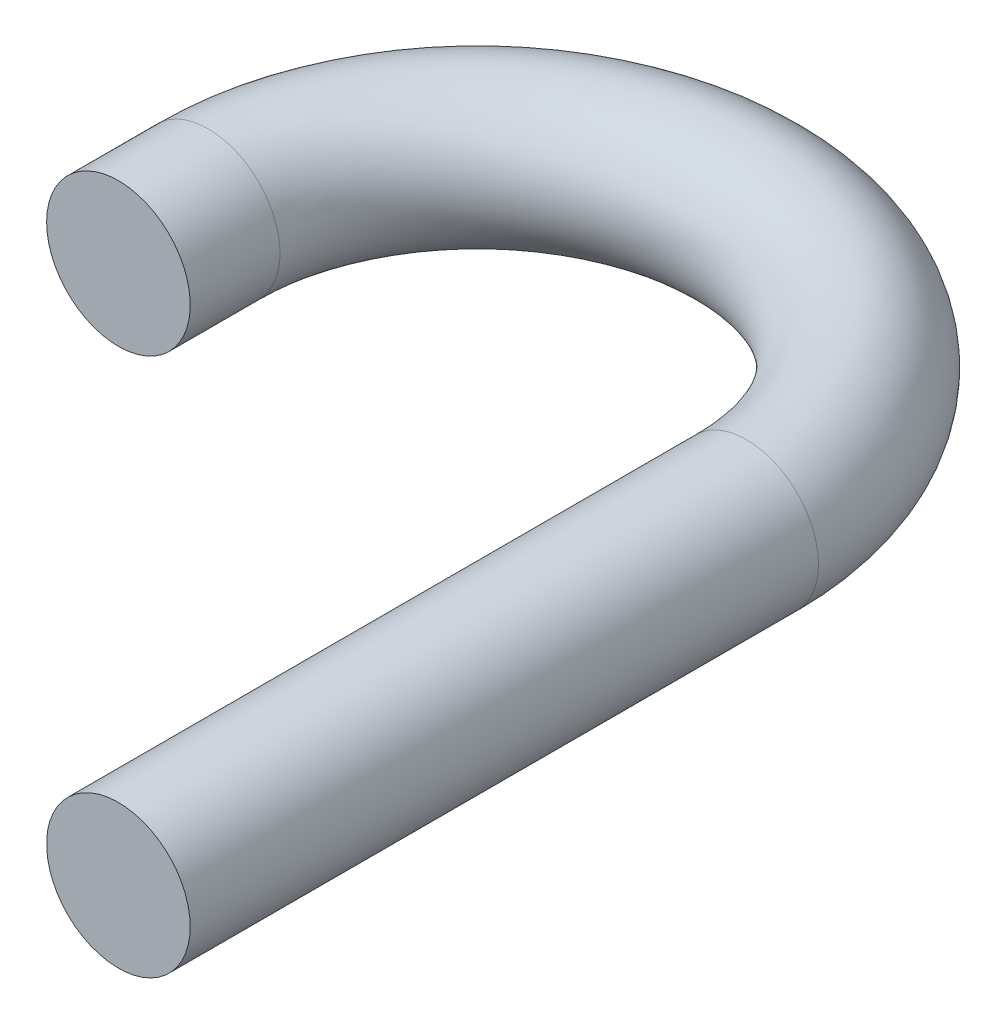
SolidWorks part; units mm, degrees
ref_plane "Front Plane" through (0, 0, 0) normal (0, 0, 1) x (1, 0, 0)
ref_plane "Top Plane" through (0, 0, 0) normal (0, 1, 0) x (1, 0, 0)
ref_plane "Right Plane" through (0, 0, 0) normal (1, 0, 0) x (0, 0, -1)
sketch "Sketch1" plane through (0, 0, 0) normal (0, 0, 1) x (1, 0, 0)
  circle A0 centre (0, 0) radius 8
  dimension "D1" = 16
sketch "Sketch2" plane through (0, 0, 0) normal (0, 1, 0) x (1, 0, 0)
  line L0 (0, 0) -> (0, 70)
  line L1 (-60, 70) -> (-60, 60)
  arc A0 (0, 70) -> (-60, 70) centre (-30, 70) ccw
  dimension "D2" = 30
  dimension "D1" = 70
  dimension "D3" = 10
sweep "Sweep1" add profiles "Sketch1" path "Sketch2"
sketch "Sketch3" plane through (0, 0, 0) normal (0, 0, 1) x (1, 0, 0)
  line L0 (0, 0) -> (0, 6.8457) construction
  line L1 (0, 0) -> (6.4316, 0) construction
